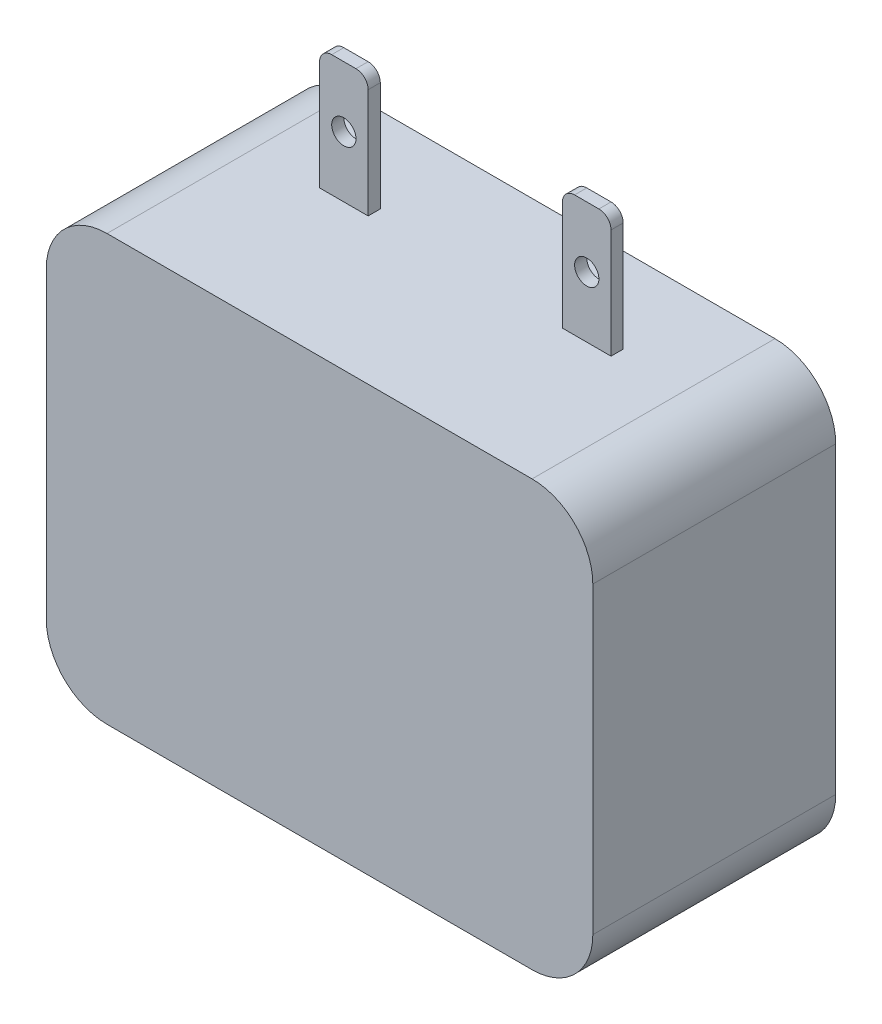
from build123d import *

# Parameters (mm, degrees)
BOSS_EXTRUDE1_DEPTH = 10
SKETCH3_R           = 1
BOSS_EXTRUDE2_DEPTH = 1
SKETCH4_R           = 1
CUT_EXTRUDE1_DEPTH  = 1


with BuildPart() as part:
    # Sketch1 → Boss-Extrude1 (new, symmetric)
    with BuildSketch(Plane.XY):
        with BuildLine():
            Line((-17.5, -17.5), (17.5, -17.5))
            ThreePointArc((17.5, -17.5), (21.035533906, -16.035533906), (22.5, -12.5))
            Line((22.5, -12.5), (22.5, 12.5))
            ThreePointArc((22.5, 12.5), (21.035533906, 16.035533906), (17.5, 17.5))
            Line((17.5, 17.5), (-17.5, 17.5))
            ThreePointArc((-17.5, 17.5), (-21.035533906, 16.035533906), (-22.5, 12.5))
            Line((-22.5, 12.5), (-22.5, -12.5))
            ThreePointArc((-22.5, -12.5), (-21.035533906, -16.035533906), (-17.5, -17.5))
        make_face()
    extrude(amount=BOSS_EXTRUDE1_DEPTH, both=True)

    # Sketch3 → Boss-Extrude2 (add)
    # profile 1 of 3: a face of its own
    with BuildSketch(Plane(origin=(0, 0, -3), x_dir=(-1, 0, 0), z_dir=(0, 0, -1))):
        with BuildLine():
            Line((-8, 17.5), (-12, 17.5))
            Line((-12, 17.5), (-12, 26.5))
            ThreePointArc((-12, 26.5), (-11.707106781, 27.207106781), (-11, 27.5))
            Line((-11, 27.5), (-9, 27.5))
            ThreePointArc((-9, 27.5), (-8.292893219, 27.207106781), (-8, 26.5))
            Line((-8, 26.5), (-8, 17.5))
        make_face()
    # profile 2 of 3: a face of its own
    with BuildSketch(Plane(origin=(0, 0, -3), x_dir=(-1, 0, 0), z_dir=(0, 0, -1))):
        with BuildLine():
            Line((8, 17.5), (12, 17.5))
            Line((12, 17.5), (12, 26.5))
            ThreePointArc((12, 26.5), (11.707106781, 27.207106781), (11, 27.5))
            Line((11, 27.5), (9, 27.5))
            ThreePointArc((9, 27.5), (8.292893219, 27.207106781), (8, 26.5))
            Line((8, 26.5), (8, 17.5))
        make_face()
    # profile 3 of 3: a face of its own
    with BuildSketch(Plane(origin=(0, 0, -3), x_dir=(-1, 0, 0), z_dir=(0, 0, -1))):
        with BuildLine():
            Line((-2.5, -17.5), (2.5, -17.5))
            Line((2.5, -17.5), (2.5, -26.5))
            ThreePointArc((2.5, -26.5), (2.207106781, -27.207106781), (1.5, -27.5))
            Line((1.5, -27.5), (-1.5, -27.5))
            ThreePointArc((-1.5, -27.5), (-2.207106781, -27.207106781), (-2.5, -26.5))
            Line((-2.5, -26.5), (-2.5, -17.5))
        make_face()
        with Locations((0, -22.5)):
            Circle(SKETCH3_R, mode=Mode.SUBTRACT)
    extrude(amount=-BOSS_EXTRUDE2_DEPTH)

    # Sketch4 → Cut-Extrude1 (cut)
    with BuildSketch(Plane(origin=(0, 0, -3), x_dir=(-1, 0, 0), z_dir=(0, 0, -1))):
        with Locations((-10, 22.5)):
            Circle(SKETCH4_R)
        with Locations((10, 22.5)):
            Circle(SKETCH4_R)
    extrude(amount=-CUT_EXTRUDE1_DEPTH, mode=Mode.SUBTRACT)


solid = part.part
